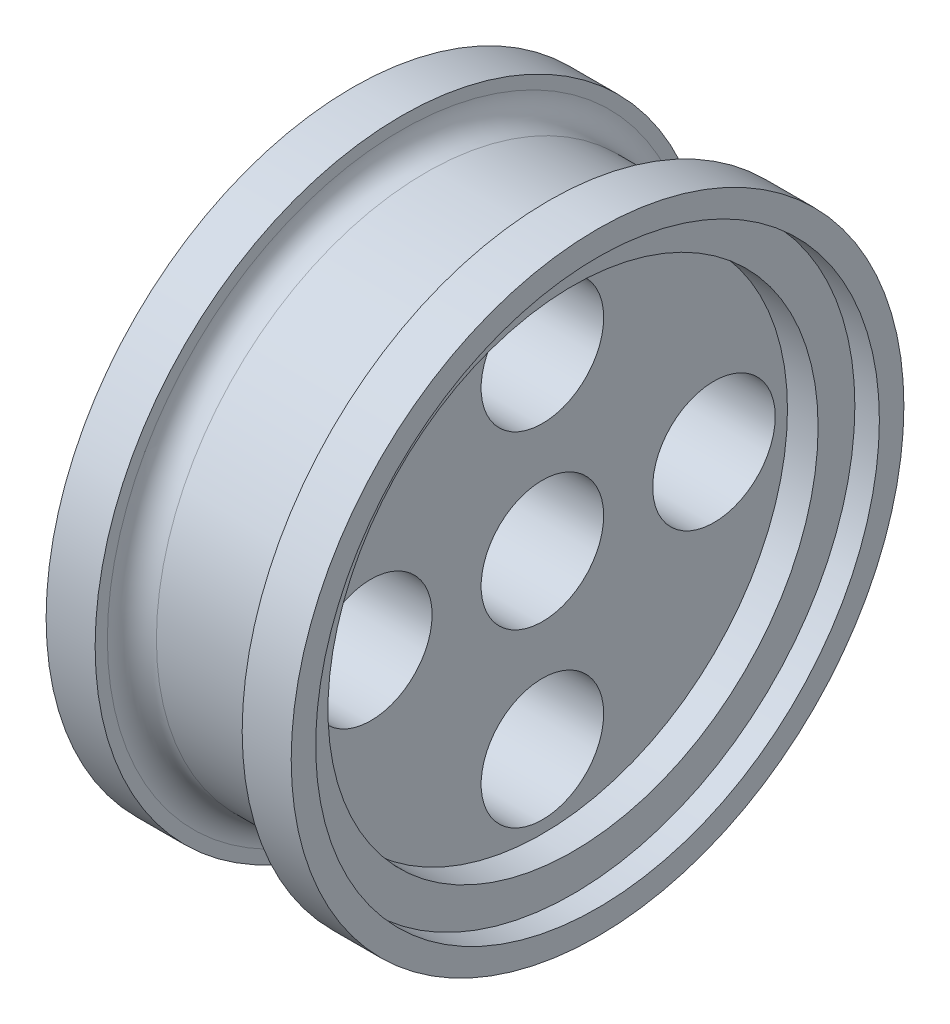
SolidWorks part; units mm, degrees
ref_plane "Front Plane" through (0, 0, 0) normal (0, 0, 1) x (1, 0, 0)
ref_plane "Top Plane" through (0, 0, 0) normal (0, 1, 0) x (1, 0, 0)
ref_plane "Right Plane" through (0, 0, 0) normal (1, 0, 0) x (0, 0, -1)
sketch "Sketch1" plane through (0, 0, 0) normal (0, 0, 1) x (1, 0, 0)
  line L0 (0, 0) -> (0, 10.9628) construction
  line L1 (0, 0) -> (5, 0)
  line L2 (5, 0) -> (5, 12.5)
  line L3 (5, 12.5) -> (3, 12.5)
  line L4 (3, 12.5) -> (3, 12)
  line L5 (2, 11) -> (0, 11)
  line L6 (0, 0) -> (0, 11)
  arc A0 (3, 12) -> (2, 11) centre (2, 12) cw
  dimension "D5" = 1
  dimension "D1" = 5
  dimension "D2" = 3
  dimension "D3" = 11
  dimension "D4" = 12.5
revolve "Revolve1" add sketch "Sketch1" angle 360 about L1
mirror "Mirror1" about plane through (0, 0, 0) normal (1, 0, 0) of "Revolve1"
sketch "Sketch2" plane through (5, 0, 0) normal (1, 0, 0) x (0, 0, -1)
  circle A0 centre (0, 0) radius 11.5
  dimension "D1" = 23
extrude "Cut-Extrude1" cut sketch "Sketch2" against normal blind 1
sketch "Sketch3" plane through (4, 0, 0) normal (1, 0, 0) x (0, 0, -1)
  circle A0 centre (0, 0) radius 10
  dimension "D1" = 20
extrude "Cut-Extrude2" cut sketch "Sketch3" against normal blind 1.25
mirror "Mirror3" about plane through (0, 0, 0) normal (1, 0, 0) of "Cut-Extrude1", "Cut-Extrude2"
sketch "Sketch4" plane through (2.75, 0, 0) normal (1, 0, 0) x (0, 0, -1)
  circle A0 centre (0, 0) radius 7 construction
  circle A1 centre (0, 7) radius 2.5
  circle A2 centre (7, 0) radius 2.5
  circle A3 centre (0, -7) radius 2.5
  circle A4 centre (-7, 0) radius 2.5
  circle A5 centre (0, 0) radius 2.5
  point P14 (0, 0)
  dimension "D1" = 14
  dimension "D2" = 5
  dimension "D4" = 5
  dimension "D3" = 4
extrude "Cut-Extrude3" cut sketch "Sketch4" against normal blind 8.5
